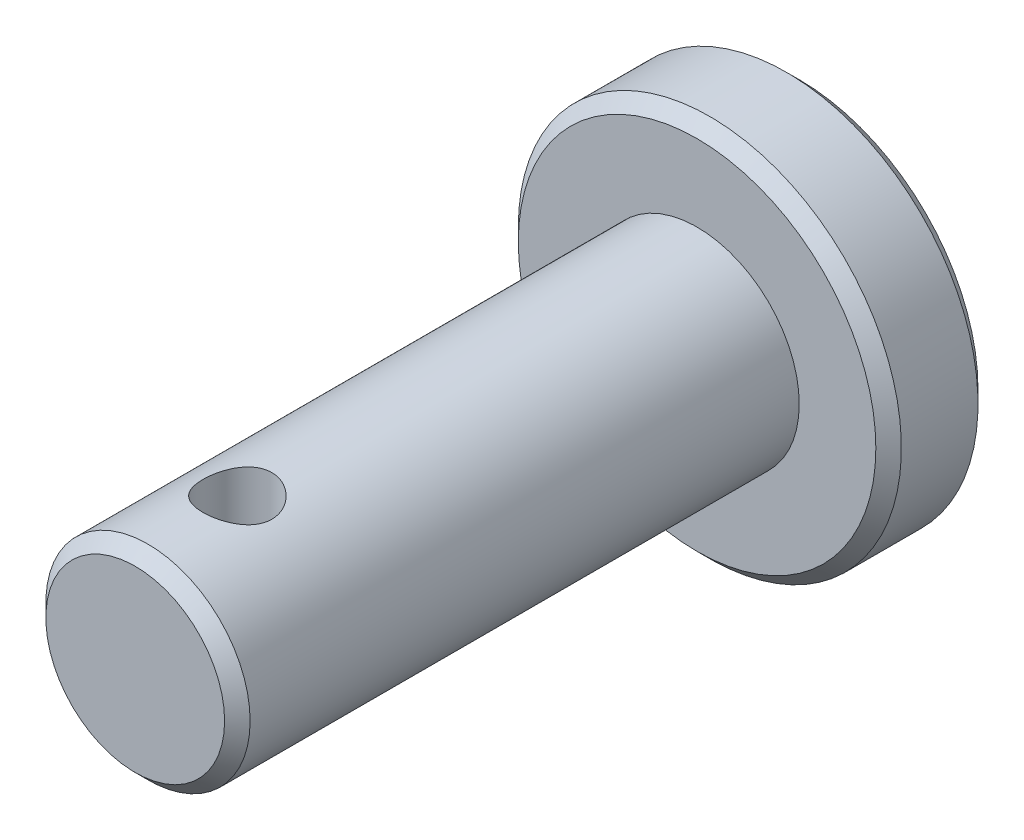
SolidWorks part; units mm, degrees
material "国产6061 "
ref_plane "Front Plane" through (0, 0, 0) normal (0, 0, 1) x (1, 0, 0)
ref_plane "Top Plane" through (0, 0, 0) normal (0, 1, 0) x (1, 0, 0)
ref_plane "Right Plane" through (0, 0, 0) normal (1, 0, 0) x (0, 0, -1)
sketch "Sketch1" plane through (0, 0, 0) normal (0, 0, 1) x (1, 0, 0)
  circle A0 centre (0, 0) radius 4
  dimension "D1" = 8
extrude "Boss-Extrude1" add sketch "Sketch1" along normal blind 22
sketch "Sketch2" plane through (0, 0, 0) normal (0, 0, -1) x (-1, 0, 0)
  circle A0 centre (0, 0) radius 7.5
  dimension "D1" = 15
extrude "Boss-Extrude2" add sketch "Sketch2" along normal blind 4
sketch "Sketch3" plane through (0, 0, 0) normal (0, 1, 0) x (1, 0, 0)
  line L0 (-4, -22) -> (4, -22) construction
  circle A0 centre (0, -18) radius 1.35
  dimension "D1" = 2.7
  dimension "D2" = 4
extrude "Cut-Extrude1" cut sketch "Sketch3" against normal through all both and the other way through all
chamfer "Chamfer1" distance 0.5 angle 45 3 edges at (4, 0, 22) (-7.5, 0, -4) (-7.5, 0, 0)
